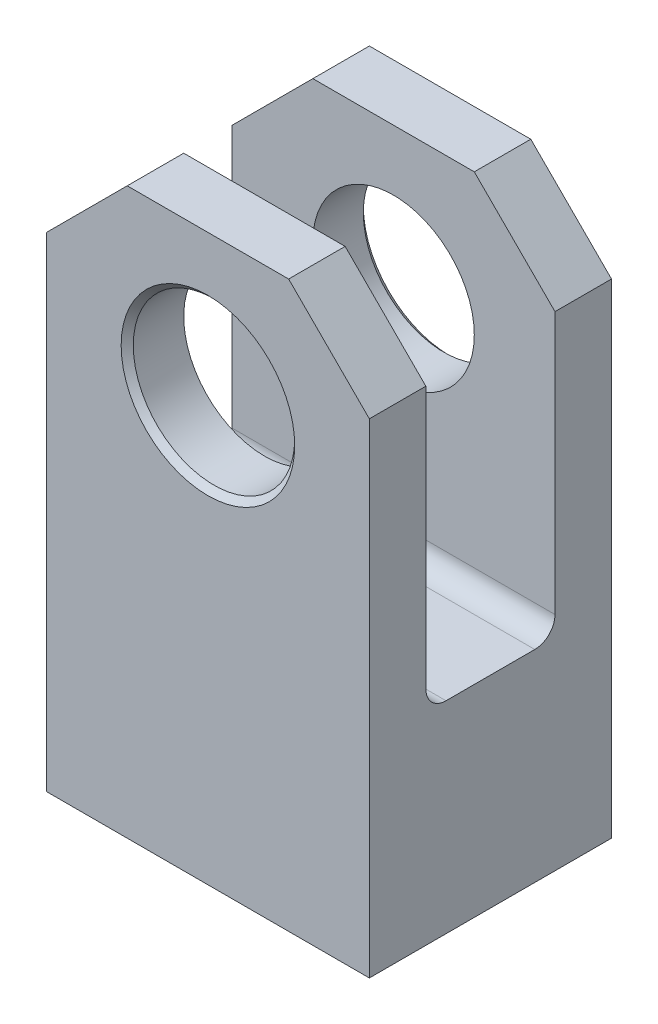
SolidWorks part; units mm, degrees
material "45#"
ref_plane "Front Plane" through (0, 0, 0) normal (0, 0, 1) x (1, 0, 0)
ref_plane "Top Plane" through (0, 0, 0) normal (0, 1, 0) x (1, 0, 0)
ref_plane "Right Plane" through (0, 0, 0) normal (1, 0, 0) x (0, 0, -1)
sketch "Sketch2" plane through (0, 0, 0) normal (0, 0, 1) x (1, 0, 0)
  line L1 (40, -70) -> (-40, -70)
  line L2 (40, -70) -> (40, 70)
  line L3 (40, 70) -> (-40, 70)
  line L4 (-40, -70) -> (-40, 70)
  line L5 (40, -70) -> (-40, 70) construction
  line L6 (40, 70) -> (-40, -70) construction
  point P0 (0, 0)
  dimension "D1" = 140
  dimension "D2" = 80
extrude "Boss-Extrude1" add sketch "Sketch2" along normal mid plane 60
chamfer "Chamfer1" distance 20 angle 45 2 edges at (40, 70, 0) (-40, 70, 0)
sketch "Sketch3" plane through (-40, 0, 0) normal (-1, 0, 0) x (0, 0, 1)
  line L0 (-30, 70) -> (30, 70) construction
  line L1 (16, 160) -> (-16, 160)
  line L2 (16, 160) -> (16, -20)
  line L3 (16, -20) -> (-16, -20)
  line L4 (-16, 160) -> (-16, -20)
  line L5 (16, 160) -> (-16, -20) construction
  line L6 (16, -20) -> (-16, 160) construction
  line L7 (30, -70) -> (-30, -70) construction
  point P0 (0, 70)
  dimension "D1" = 32
  dimension "D2" = 50
extrude "Cut-Extrude1" cut sketch "Sketch3" against normal through all both and the other way through all
fillet "Fillet1" radius 5 2 edges at (0, -20, 16) (0, -20, -16)
sketch "Sketch4" plane through (0, 0, 30) normal (0, 0, 1) x (1, 0, 0)
  line L0 (0, -70) -> (0, 35) construction
  line L1 (-40, -70) -> (40, -70) construction
  circle A0 centre (0, 35) radius 20
  dimension "D2" = 40
  dimension "D1" = 105
extrude "Cut-Extrude2" cut sketch "Sketch4" against normal through all both and the other way through all
chamfer "Chamfer2" distance 1.5 angle 45 2 edges at (20, 35, 30) (20, 35, -30)
hole_wizard "M24 Tapped Hole1" positions "Sketch5" profile "Sketch6" tap size "M24" standard "GB" end condition up to next
sketch "Sketch5" plane through (0, -20, 0) normal (0, 1, 0) x (1, 0, 0)
  point P0 (0, 0)
sketch "Sketch6" plane through (0, -20, 0) normal (1, 0, 0) x (0, 0, 1)
  line L0 (0, 0) -> (0, 50)
  line L1 (0, 50) -> (10.5, 50)
  line L2 (10.5, 50) -> (10.5, 0)
  line L5 (10.5, 0) -> (0, 0)
  line L11 (0, -6.35) -> (0, 107.95) construction
  dimension "通孔螺纹孔钻头直径" = 21
  dimension "通孔螺纹孔钻头深度" = 50
cosmetic thread "Tapped hole thread1" parameters "D2"=24
